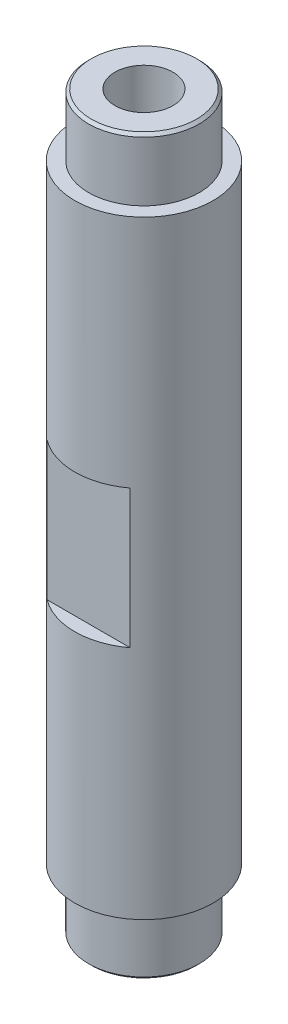
SolidWorks part; units mm, degrees
material "A6061"
ref_plane "前视基准面" through (0, 0, 0) normal (0, 0, 1) x (1, 0, 0)
ref_plane "上视基准面" through (0, 0, 0) normal (0, 1, 0) x (1, 0, 0)
ref_plane "右视基准面" through (0, 0, 0) normal (1, 0, 0) x (0, 0, -1)
sketch "Sketch1" plane through (0, 0, 0) normal (1, 0, 0) x (0, 0, -1)
  line L1 (-5, 26.5) -> (0, 26.5)
  line L2 (-5, 26.5) -> (-5, -26.5)
  line L3 (-5, -26.5) -> (0, -26.5)
  line L4 (0, 26.5) -> (0, -26.5)
  dimension "D1" = 53
  dimension "D2" = 5
revolve "Revolve1" add sketch "Sketch1" angle 360 about L4
hole_wizard "M5 Tapped Hole1" positions "Sketch3" profile "Sketch2" tap size "M5" standard "GB"
sketch "Sketch3" plane through (0, 26.5, 0) normal (0, 1, 0) x (1, 0, 0)
  point P0 (0, 0)
cosmetic thread "Cosmetic Thread1" parameters "D1"=8, "D2"=5
sketch "Sketch2" plane through (0, 26.5, 0) normal (1, 0, 0) x (0, 0, 1)
  line L0 (0, 0) -> (0, 11.6618)
  line L1 (0, 11.6618) -> (2.1, 10.4)
  line L2 (2.1, 10.4) -> (2.1, 0)
  line L5 (2.1, 0) -> (0, 0)
  line L10 (0, 11.6618) -> (-2.1, 10.4) construction
  line L11 (0, -6.35) -> (0, 107.95) construction
  dimension "螺纹孔钻头直径" = 4.2
  dimension "螺纹孔钻头深度" = 10.4
  dimension "导头角度" = 118
mirror "Mirror1" about plane through (0, 0, 0) normal (0, 1, 0) of "M5 Tapped Hole1"
sketch "Sketch4" plane through (0, -26.5, 0) normal (0, -1, 0) x (1, 0, 0)
  circle A0 centre (0, 0) radius 4
  dimension "D1" = 8
extrude "Extrude1" cut sketch "Sketch4" against normal blind 4.5 flip side to cut
sketch "Sketch5" plane through (0, 26.5, 0) normal (0, 1, 0) x (1, 0, 0)
  circle A0 centre (0, 0) radius 4
  dimension "D1" = 8
extrude "Extrude2" cut sketch "Sketch5" against normal blind 4.5 flip side to cut
sketch "Sketch6" plane through (0, 0, 0) normal (1, 0, 0) x (0, 0, -1)
  line L0 (-4, 0) -> (4, 0) construction
  line L1 (-11.2311, 5) -> (-4, 5)
  line L2 (-11.2311, 5) -> (-11.2311, -5)
  line L3 (-11.2311, -5) -> (-4, -5)
  line L4 (-4, 5) -> (-4, -5)
  line L5 (6.6065, 5) -> (4, 5)
  line L6 (6.6065, 5) -> (6.6065, -5)
  line L7 (6.6065, -5) -> (4, -5)
  line L8 (4, 5) -> (4, -5)
  dimension "D1" = 8
  dimension "D2" = 10
extrude "Extrude3" cut sketch "Sketch6" against normal through all and the other way through all
chamfer "Chamfer1" distance 0.2 angle 45 2 edges at (0, -26.5, -4) (0, 26.5, 4)
